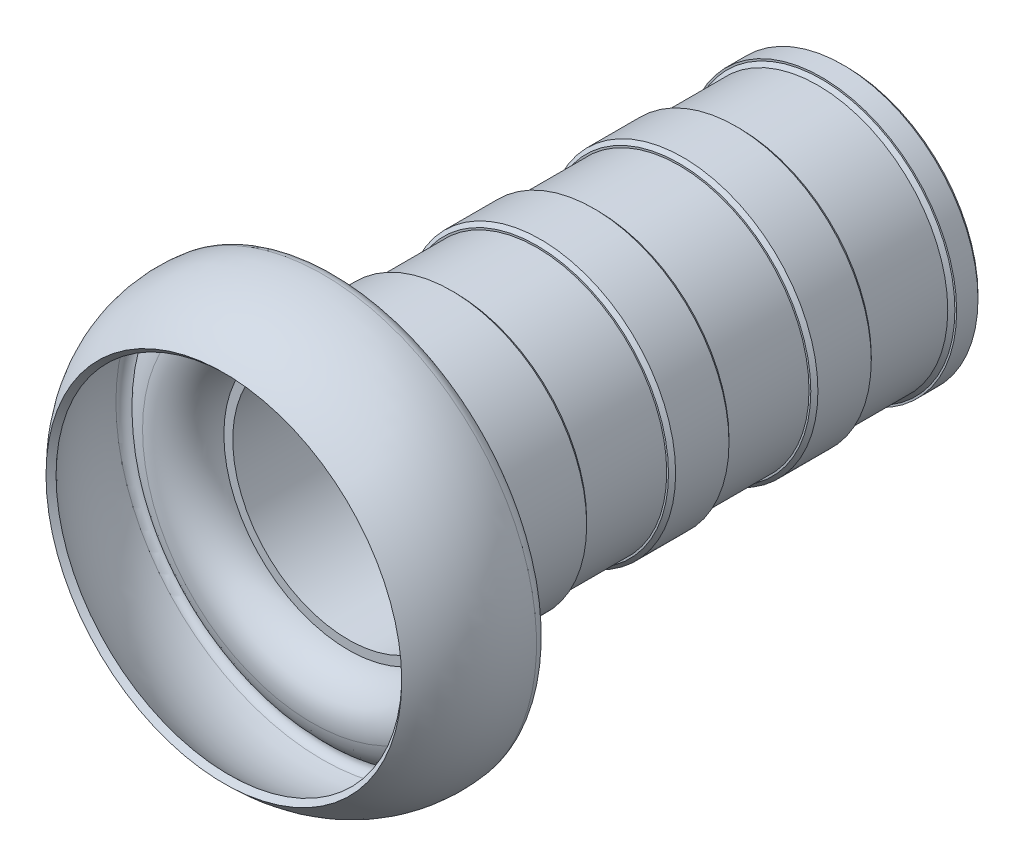
SolidWorks part; units mm, degrees
ref_plane "前视基准面" through (0, 0, 0) normal (0, 0, 1) x (1, 0, 0)
ref_plane "上视基准面" through (0, 0, 0) normal (0, 1, 0) x (1, 0, 0)
ref_plane "右视基准面" through (0, 0, 0) normal (1, 0, 0) x (0, 0, -1)
sketch "草图1" plane through (0, 0, 0) normal (0, 0, 1) x (1, 0, 0)
  circle A0 centre (0, 0) radius 38
  circle A1 centre (0, 0) radius 32.5
  dimension "D1" = 76
  dimension "D2" = 5.5
extrude "凸台-拉伸1" add sketch "草图1" along normal blind 140
chamfer "倒角1" distance 1 angle 45 1 edges at (38, 0, 140)
ref_plane "基准面1" through (0, 0, 110) normal (0, 0, 1) x (1, 0, 0)
sketch "草图2" plane through (0, 0, 110) normal (0, 0, 1) x (1, 0, 0)
  circle A0 centre (0, 0) radius 38
  circle A1 centre (0, 0) radius 36.5
  dimension "D1" = 76
  dimension "D2" = 73
extrude "切除-拉伸1" cut sketch "草图2" against normal blind 23
pattern_linear "阵列(线性)1" count 3 spacing 40 along (0, 0, -1) of "切除-拉伸1"
chamfer "倒角2" distance 1 angle 45 7 edges at (38, 0, 0) (36.5, 0, 7) (38, 0, 30) (38, 0, 47) (38, 0, 70) (38, 0, 87) (38, 0, 110)
sketch "草图3" plane through (0, 0, 0) normal (0, 1, 0) x (1, 0, 0)
  line L0 (0, -140) -> (0, -175) construction
  line L1 (-37, -140) -> (37, -140) construction
  line L2 (0, -140) -> (37, -140) construction
  line L3 (50, -175) -> (48.6148, -173.5574)
  line L4 (35, -140) -> (37, -140)
  line L5 (2, -142) -> (35.193, -142) construction
  line L6 (2, -142) -> (2, -175) construction
  arc A0 (37, -140) -> (47.213, -148.274) centre (45.4581, -140) ccw
  arc A1 (47.213, -148.274) -> (54.2052, -143.5436) centre (44.8856, -137.3009) ccw
  arc A2 (54.2052, -143.5436) -> (60, -147.0986) centre (55.7011, -147.6056) cw
  arc A3 (60, -147.0986) -> (50, -175) centre (26.9514, -150.9965) cw
  arc A4 (35, -140) -> (47.6279, -150.2305) centre (45.4581, -140) ccw
  arc A5 (47.6279, -150.2305) -> (55.4112, -145.295) centre (44.8856, -137.3009) ccw
  arc A6 (55.4112, -145.295) -> (58.0138, -147.3328) centre (55.7011, -147.6056) cw
  arc A7 (58.0138, -147.3328) -> (48.6148, -173.5574) centre (26.9514, -150.9965) cw
  arc A8 (35.193, -142) -> (47.6279, -150.2305) centre (45.4581, -140) ccw construction
  dimension "D1" = 35
  dimension "D2" = 60
  dimension "D3" = 50
  dimension "D4" = 2
revolve "旋转1" add sketch "草图3" angle 360 about L0
